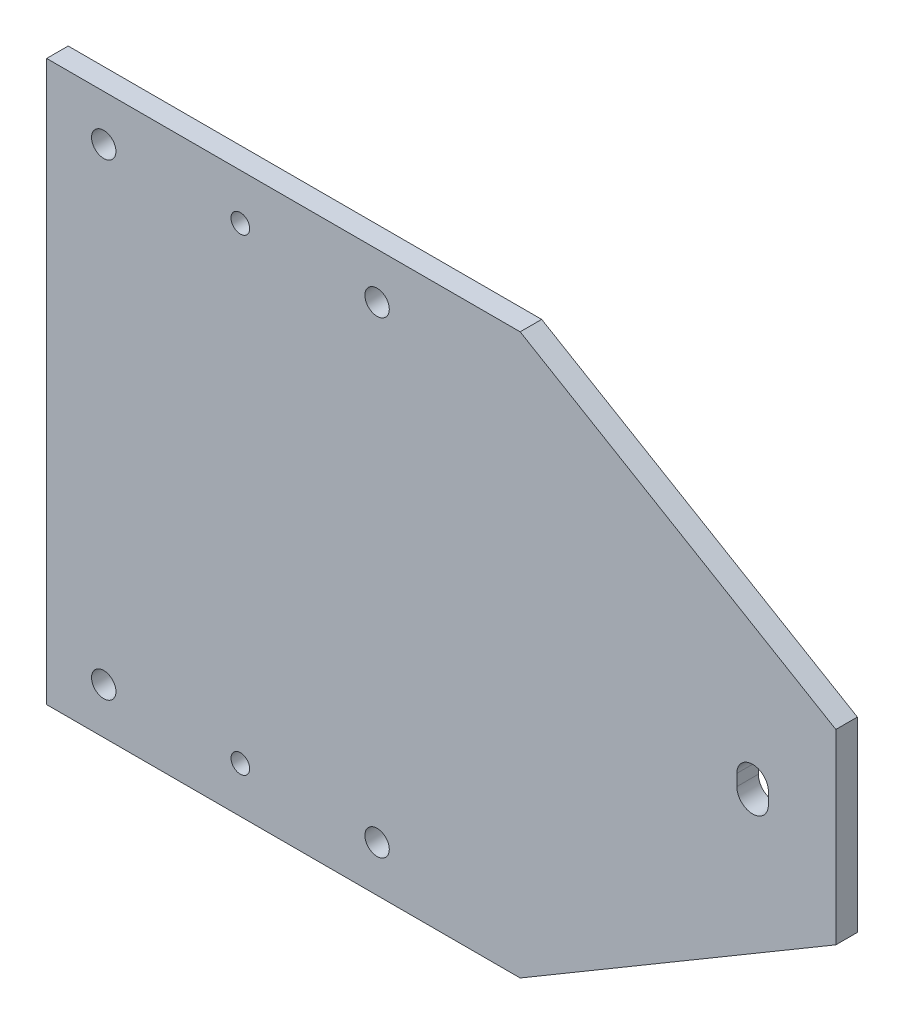
SolidWorks part; units mm, degrees
material "1023 碳钢板 (SS)"
ref_plane "前视基准面" through (0, 0, 0) normal (0, 0, 1) x (1, 0, 0)
ref_plane "上视基准面" through (0, 0, 0) normal (0, 1, 0) x (1, 0, 0)
ref_plane "右视基准面" through (0, 0, 0) normal (1, 0, 0) x (0, 0, -1)
sketch "草图1" plane through (0, 0, 0) normal (0, 0, 1) x (1, 0, 0)
  line L1 (275, 195) -> (-275, 195)
  line L2 (275, 195) -> (275, -195)
  line L3 (275, -195) -> (-275, -195)
  line L4 (-275, 195) -> (-275, -195)
  line L5 (275, 195) -> (-275, -195) construction
  line L6 (275, -195) -> (-275, 195) construction
  point P0 (0, 0)
  dimension "D1" = 550
  dimension "D2" = 390
extrude "凸台-拉伸1" add sketch "草图1" along normal blind 15
sketch "草图2" plane through (0, 0, 15) normal (0, 0, 1) x (1, 0, 0)
  line L0 (-275, 195) -> (-275, -195) construction
  line L1 (55, 195) -> (275, 65)
  line L2 (275, 195) -> (-275, 195) construction
  line L3 (275, -195) -> (275, 195) construction
  line L4 (275, 65) -> (275, 195)
  line L5 (275, 195) -> (55, 195)
  line L6 (55, -195) -> (275, -65)
  line L7 (-275, -195) -> (275, -195) construction
  line L8 (275, -65) -> (275, -195)
  line L9 (275, -195) -> (55, -195)
  line L10 (217, 4) -> (217, -4) construction
  line L11 (228, 4) -> (228, -4)
  line L12 (206, 4) -> (206, -4)
  circle A0 centre (-235.2, 163) radius 8.5
  circle A1 centre (-235.2, -163) radius 8.5
  circle A2 centre (-140, -163) radius 6.5
  circle A3 centre (-44.7, -163) radius 8.5
  circle A4 centre (-140, 163) radius 6.5
  circle A5 centre (-44.7, 163) radius 8.5
  arc A6 (228, 4) -> (206, 4) centre (217, 4) ccw
  arc A7 (206, -4) -> (228, -4) centre (217, -4) ccw
  point P22 (217, 0)
  point P36 (0, 0)
  dimension "D5" = 17
  dimension "D6" = 13
  dimension "D7" = 39.8
  dimension "D12" = 8
  dimension "D13" = 11
  dimension "D1" = 326
  dimension "D2" = 135
  dimension "D3" = 190.5
  dimension "D4" = 163
  dimension "D8" = 130
  dimension "D9" = 220
  dimension "D10" = 220
  dimension "D11" = 130
  dimension "D14" = 58
extrude "切除-拉伸1" cut sketch "草图2" against normal blind 15
